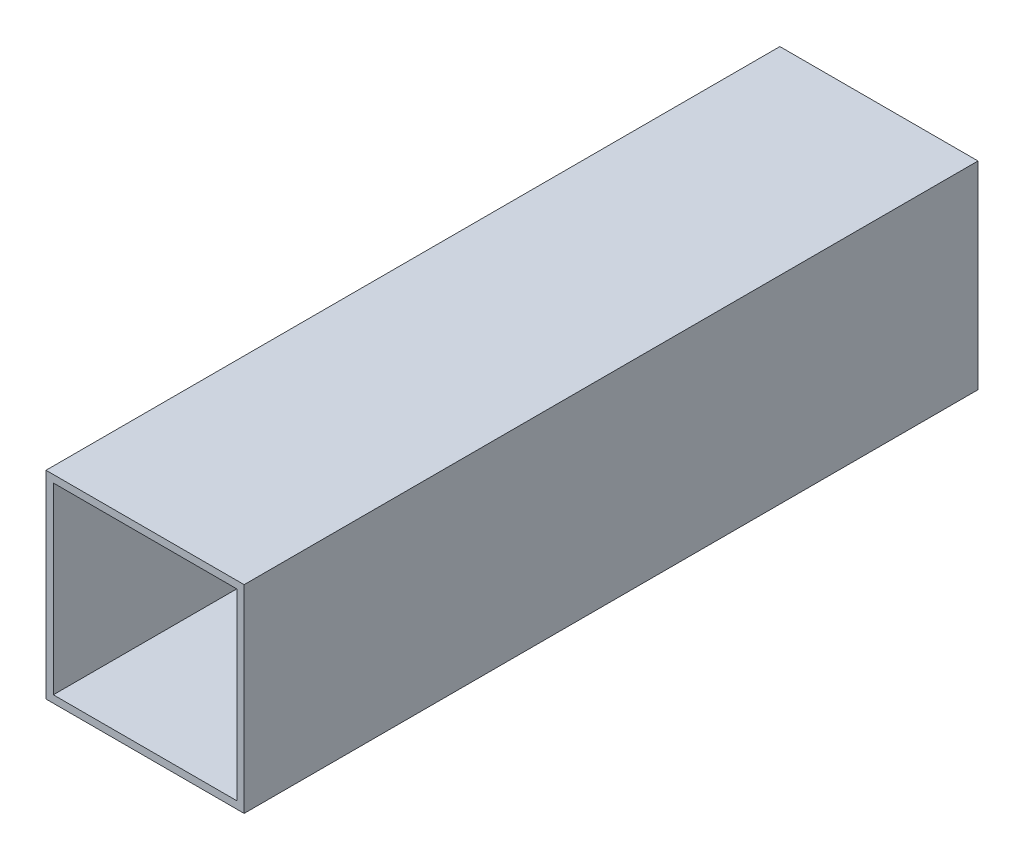
from build123d import *

# Parameters (mm, degrees)
SKETCH1_W           = 270
SKETCH1_H           = 270
SKETCH1_W_2         = 250
SKETCH1_H_2         = 250
EXTRUDE_THIN1_DEPTH = 1000


with BuildPart() as part:
    # Sketch1 → Extrude-Thin1 (new body)
    with BuildSketch(Plane.XY):
        Rectangle(SKETCH1_W, SKETCH1_H)
        Rectangle(SKETCH1_W_2, SKETCH1_H_2, mode=Mode.SUBTRACT)
    extrude(amount=EXTRUDE_THIN1_DEPTH)


solid = part.part
